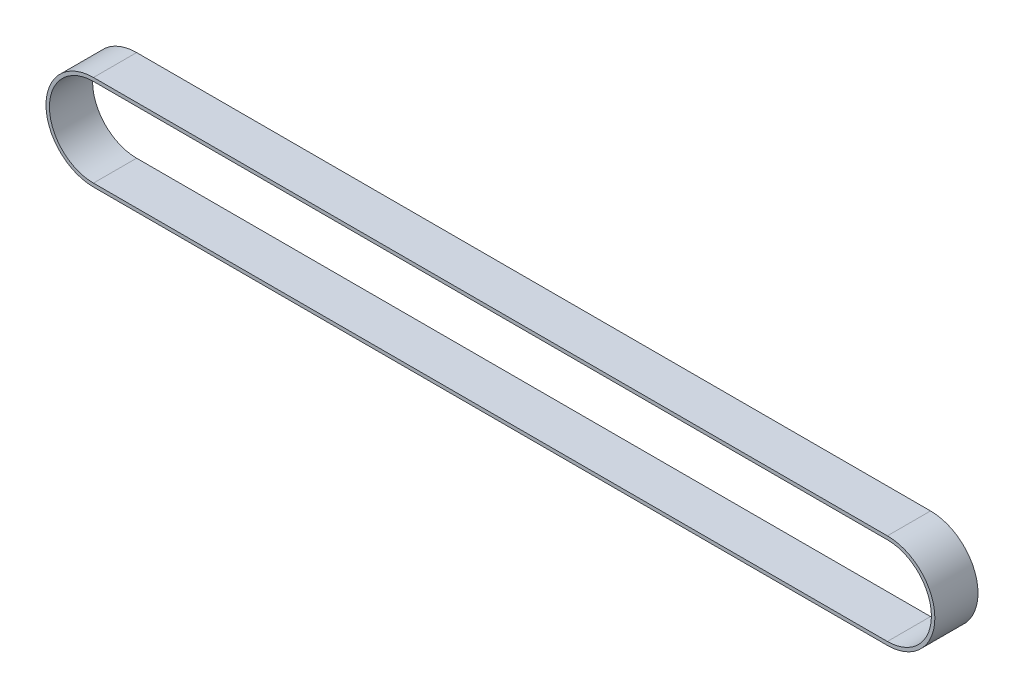
SolidWorks part; units mm, degrees
ref_plane "前视基准面" through (0, 0, 0) normal (0, 0, 1) x (1, 0, 0)
ref_plane "上视基准面" through (0, 0, 0) normal (0, 1, 0) x (1, 0, 0)
ref_plane "右视基准面" through (0, 0, 0) normal (1, 0, 0) x (0, 0, -1)
sketch "草图1" plane through (0, 0, 0) normal (0, 0, 1) x (1, 0, 0)
  line L0 (-230, 0) -> (230, 0) construction
  line L1 (-230, 25.5) -> (230, 25.5)
  line L2 (-230, -25.5) -> (230, -25.5)
  arc A0 (-230, 25.5) -> (-230, -25.5) centre (-230, 0) ccw
  arc A1 (230, -25.5) -> (230, 25.5) centre (230, 0) ccw
  point P2 (0, 0)
  dimension "D1" = 25.5
  dimension "D2" = 460
extrude "拉伸-薄壁1" add sketch "草图1" along normal blind 25 thin thin type one direction wall 2
